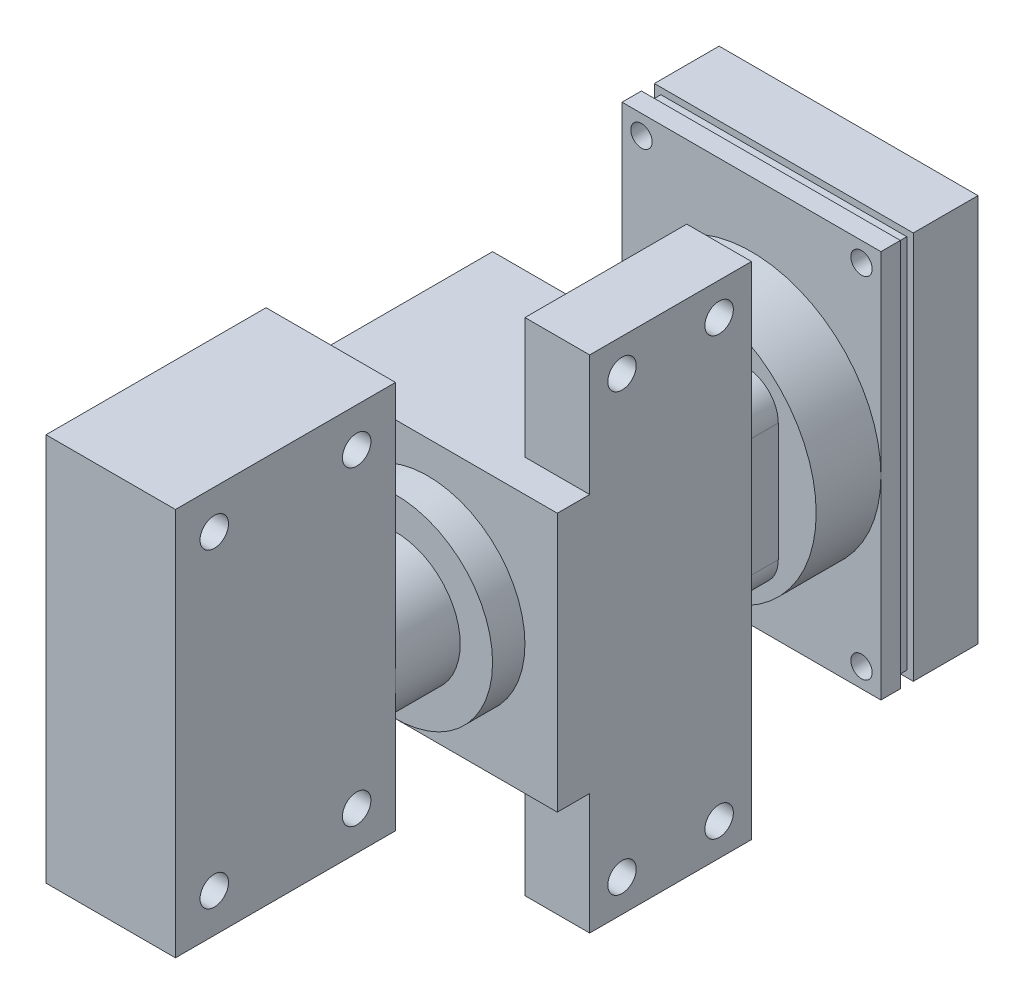
SolidWorks part; units mm, degrees
ref_plane "前视基准面" through (0, 0, 0) normal (0, 0, 1) x (1, 0, 0)
ref_plane "上视基准面" through (0, 0, 0) normal (0, 1, 0) x (1, 0, 0)
ref_plane "右视基准面" through (0, 0, 0) normal (1, 0, 0) x (0, 0, -1)
sketch "草图1" plane through (0, 0, 0) normal (0, 0, 1) x (1, 0, 0)
  line L1 (20, -30) -> (-20, -30)
  line L2 (20, -30) -> (20, 30)
  line L3 (20, 30) -> (-20, 30)
  line L4 (-20, -30) -> (-20, 30)
  line L5 (20, -30) -> (-20, 30) construction
  line L6 (20, 30) -> (-20, -30) construction
  point P0 (0, 0)
  dimension "D1" = 40
  dimension "D2" = 60
extrude "凸台-拉伸1" add sketch "草图1" along normal blind 10
sketch "草图2" plane through (0, 0, 10) normal (0, 0, 1) x (1, 0, 0)
  line L8 (-19, 29) -> (-19, -29)
  line L9 (-19, -29) -> (19, -29)
  line L10 (19, -29) -> (19, 29)
  line L11 (19, 29) -> (-19, 29)
  line L12 (-19, 29) -> (-19, -29)
  line L13 (-19, -29) -> (19, -29)
  line L14 (19, -29) -> (19, 29)
  line L15 (19, 29) -> (-19, 29)
  dimension "D1" = 1
extrude "凸台-拉伸2" add sketch "草图2" along normal blind 2
sketch "草图3" plane through (0, 0, 12) normal (0, 0, 1) x (1, 0, 0)
  line L4 (-20, 30) -> (-20, -30)
  line L5 (-20, -30) -> (20, -30)
  line L6 (20, -30) -> (20, 30)
  line L7 (20, 30) -> (-20, 30)
  line L8 (-20, 30) -> (-20, -30)
  line L9 (-20, -30) -> (20, -30)
  line L10 (20, -30) -> (20, 30)
  line L11 (20, 30) -> (-20, 30)
  dimension "D1" = 0
extrude "凸台-拉伸3" add sketch "草图3" along normal blind 3
sketch "草图4" plane through (0, 0, 15) normal (0, 0, 1) x (1, 0, 0)
  circle A0 centre (0, 0) radius 20
  dimension "D1" = 40
extrude "凸台-拉伸4" add sketch "草图4" along normal blind 10
sketch "草图5" plane through (0, 0, 25) normal (0, 0, 1) x (1, 0, 0)
  line L1 (9.1421, -14.1421) -> (-9.1421, -14.1421)
  line L2 (14.1421, -9.1421) -> (14.1421, 9.1421)
  line L3 (9.1421, 14.1421) -> (-9.1421, 14.1421)
  line L4 (-14.1421, -9.1421) -> (-14.1421, 9.1421)
  line L5 (14.1421, -14.1421) -> (-14.1421, 14.1421) construction
  line L6 (14.1421, 14.1421) -> (-14.1421, -14.1421) construction
  circle A0 centre (0, 0) radius 20 construction
  arc A1 (-14.1421, -9.1421) -> (-9.1421, -14.1421) centre (-9.1421, -9.1421) ccw
  arc A2 (9.1421, -14.1421) -> (14.1421, -9.1421) centre (9.1421, -9.1421) ccw
  arc A3 (14.1421, 9.1421) -> (9.1421, 14.1421) centre (9.1421, 9.1421) ccw
  arc A4 (-14.1421, 9.1421) -> (-9.1421, 14.1421) centre (-9.1421, 9.1421) cw
  point P0 (0, 0)
  dimension "D1" = 5
extrude "凸台-拉伸5" add sketch "草图5" along normal blind 10
sketch "草图6" plane through (0, 0, 0) normal (0, 0, -1) x (-1, 0, 0)
  line L8 (17, -27) -> (17, 27)
  line L9 (17, 27) -> (-17, 27)
  line L10 (-17, 27) -> (-17, -27)
  line L11 (-17, -27) -> (17, -27)
  line L12 (17, -27) -> (17, 27) construction
  line L13 (17, 27) -> (-17, 27) construction
  line L14 (-17, 27) -> (-17, -27) construction
  line L15 (-17, -27) -> (17, -27) construction
  circle A0 centre (17, 27) radius 1.65
  circle A1 centre (17, -27) radius 1.65
  circle A2 centre (-17, -27) radius 1.65
  circle A3 centre (-17, 27) radius 1.65
  dimension "D2" = 3.3
  dimension "D1" = 3
extrude "切除-拉伸1" cut sketch "草图6" against normal blind 20
sketch "草图7" plane through (0, 0, 35) normal (0, 0, 1) x (1, 0, 0)
  line L6 (0, 20) -> (0, 0) construction
  line L7 (0, 0) -> (20, 0) construction
  line L12 (20, -20) -> (20, 20)
  line L13 (20, 20) -> (-20, 20)
  line L14 (-20, 20) -> (-20, 10)
  line L15 (-20, 10) -> (-30, 10)
  line L16 (-30, 10) -> (-30, -20)
  line L17 (-30, -20) -> (20, -20)
  dimension "D1" = 40
  dimension "D2" = 40
  dimension "D3" = 50
  dimension "D4" = 30
  dimension "D5" = 10
extrude "凸台-拉伸6" add sketch "草图7" along normal blind 30
sketch "草图8" plane through (0, 0, 65) normal (0, 0, 1) x (1, 0, 0)
  circle A0 centre (0, 0) radius 15
  dimension "D1" = 30
extrude "凸台-拉伸7" add sketch "草图8" along normal blind 5
sketch "草图9" plane through (0, 0, 70) normal (0, 0, 1) x (1, 0, 0)
  circle A1 centre (0, 0) radius 10
  dimension "D1" = 20
extrude "凸台-拉伸8" add sketch "草图9" along normal blind 10
sketch "草图10" plane through (20, 0, 0) normal (1, 0, 0) x (0, 0, -1)
  line L0 (5.9961, 38.682) -> (-60, 38.682) construction
  line L1 (-60, 38.682) -> (-35, 38.682)
  line L2 (-60, 38.682) -> (-60, 20)
  line L3 (-60, 20) -> (-35, 20)
  line L4 (-35, 38.682) -> (-35, 20)
  line L5 (-60, 38.682) -> (-35, 20) construction
  line L6 (-60, 20) -> (-35, 38.682) construction
  line L7 (-60, -38.682) -> (-60, 38.682) construction
  line L8 (-65, -20) -> (-35, -20) construction
  line L9 (-35, -38.682) -> (-60, -38.682)
  line L10 (-35, -38.682) -> (-35, -20)
  line L11 (-35, -20) -> (-60, -20)
  line L12 (-60, -38.682) -> (-60, -20)
  line L13 (-35, -38.682) -> (-60, -20) construction
  line L14 (-35, -20) -> (-60, -38.682) construction
  line L15 (5.9961, -38.682) -> (-60, -38.682) construction
  point P0 (-47.5, 29.341)
  point P11 (-47.5, -29.341)
extrude "凸台-拉伸9" add sketch "草图10" against normal blind 10
sketch "草图11" plane through (10, 0, 0) normal (-1, 0, 0) x (0, 0, 1)
  line L28 (40, 33.682) -> (40, -33.682)
  line L29 (55, 33.682) -> (40, 33.682)
  line L30 (55, 15) -> (55, 33.682)
  line L31 (60, 15) -> (55, 15)
  line L32 (60, -15) -> (60, 15)
  line L33 (55, -15) -> (60, -15)
  line L34 (55, -33.682) -> (55, -15)
  line L35 (40, -33.682) -> (55, -33.682)
  line L36 (40, 33.682) -> (40, -33.682) construction
  line L37 (55, 33.682) -> (40, 33.682) construction
  line L38 (55, 15) -> (55, 33.682) construction
  line L39 (60, 15) -> (55, 15) construction
  line L40 (60, -15) -> (60, 15) construction
  line L41 (55, -15) -> (60, -15) construction
  line L42 (55, -33.682) -> (55, -15) construction
  line L43 (40, -33.682) -> (55, -33.682) construction
  circle A0 centre (55, 33.682) radius 2.2
  circle A1 centre (40, 33.682) radius 2.2
  circle A2 centre (40, -33.682) radius 2.2
  circle A3 centre (55, -33.682) radius 2.2
  dimension "D2" = 4.4
  dimension "D1" = 5
extrude "切除-拉伸2" cut sketch "草图11" against normal blind 10
sketch "草图12" plane through (0, 0, 80) normal (0, 0, 1) x (1, 0, 0)
  line L0 (0, 10) -> (0, 0) construction
  line L5 (-10, 40) -> (10, 40)
  line L6 (-10, 40) -> (-10, -20)
  line L7 (-10, -20) -> (10, -20)
  line L8 (10, 40) -> (10, -20)
  line L9 (-10, 40) -> (10, -20) construction
  line L10 (-10, -20) -> (10, 40) construction
  point P0 (0, 10)
  dimension "D1" = 60
  dimension "D2" = 20
  dimension "D3" = 10
extrude "凸台-拉伸10" add sketch "草图12" along normal blind 34
sketch "草图13" plane through (-10, 0, 0) normal (-1, 0, 0) x (0, 0, 1)
  line L10 (86, 34) -> (86, 0)
  line L11 (86, 0) -> (86, -14)
  line L12 (86, -14) -> (108, -14)
  line L13 (108, -14) -> (108, 34)
  line L14 (108, 34) -> (86, 34)
  line L15 (86, 34) -> (86, 0) construction
  line L16 (86, 0) -> (86, -14) construction
  line L17 (86, -14) -> (108, -14) construction
  line L18 (108, -14) -> (108, 34) construction
  line L19 (108, 34) -> (86, 34) construction
  circle A0 centre (108, 34) radius 2.2
  circle A1 centre (86, 34) radius 2.2
  circle A2 centre (108, -14) radius 2.2
  circle A3 centre (86, -14) radius 2.2
  dimension "D2" = 4.4
  dimension "D1" = 6
extrude "切除-拉伸3" cut sketch "草图13" against normal blind 35
